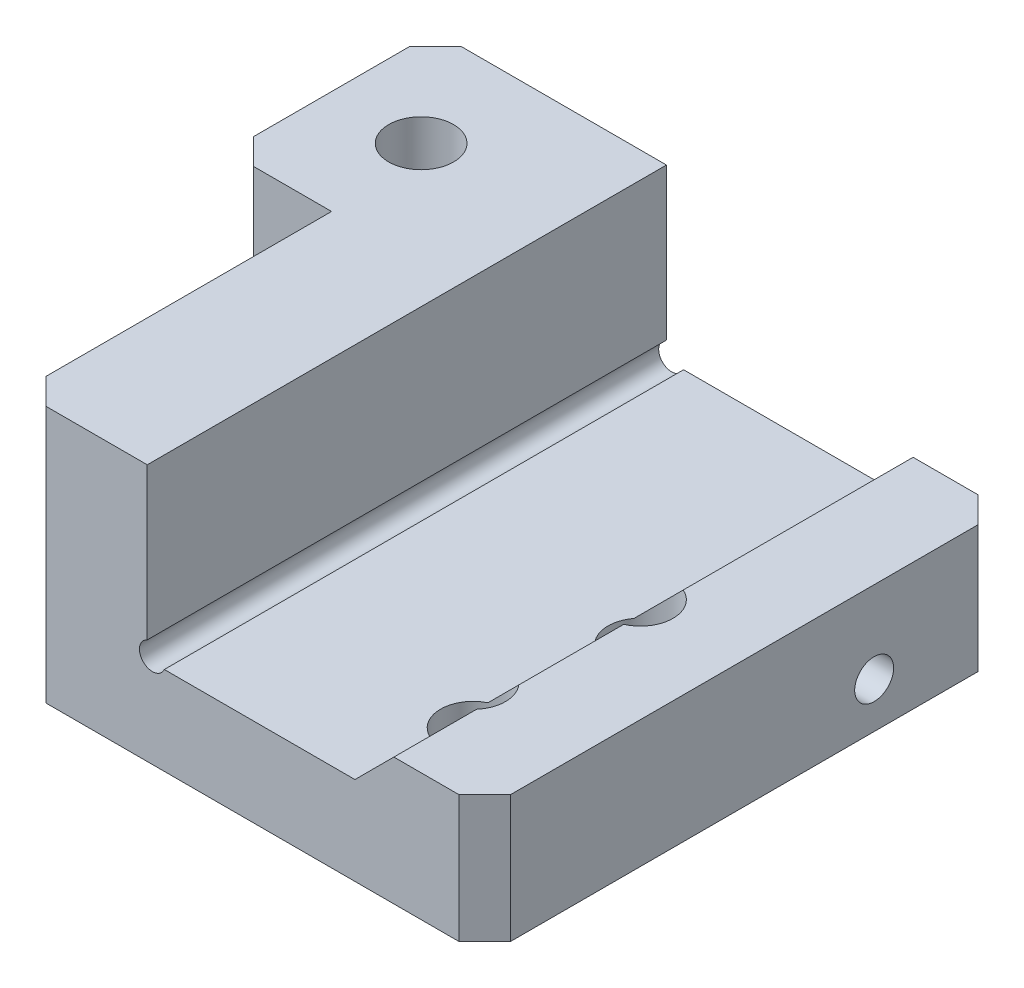
SolidWorks part; units mm, degrees
ref_plane "Front Plane" through (0, 0, 0) normal (0, 0, 1) x (1, 0, 0)
ref_plane "Top Plane" through (0, 0, 0) normal (0, 1, 0) x (1, 0, 0)
ref_plane "Right Plane" through (0, 0, 0) normal (1, 0, 0) x (0, 0, -1)
sketch "Sketch1" plane through (0, 0, 0) normal (0, 0, 1) x (1, 0, 0)
  line L0 (0, 0) -> (0, 6.5)
  line L1 (0, 6.5) -> (4.9, 6.5)
  line L2 (4.9, 6.5) -> (4.9, 4.0583)
  line L3 (5.5583, 3.4) -> (8, 3.4)
  line L4 (8, 3.4) -> (8, 0)
  line L5 (8, 0) -> (0, 0)
  arc A0 (4.9, 4.0583) -> (5.5583, 3.4) centre (5.1, 3.6) ccw
  dimension "D7" = 1
  dimension "D1" = 3.1
  dimension "D2" = 3.1
  dimension "D3" = 6.5
  dimension "D4" = 8
  dimension "D5" = 0.2
  dimension "D6" = 0.2
extrude "Boss-Extrude1" add sketch "Sketch1" along normal blind 20
other "Move Face1" face at (2.45, 6.5, 10) parameters "D1"=3.4
other "Move Face2" face at (8, 1.7, 10) parameters "D1"=9.9
sketch "Sketch10" plane through (0, 0, 0) normal (0, 0, -1) x (-1, 0, 0)
  line L0 (-17.9, 3.4) -> (-17.9, 4.9)
  line L1 (-17.9, 4.9) -> (-14.4, 4.9)
  line L2 (-14.4, 4.9) -> (-12.9, 3.4)
  line L4 (-12.9, 3.4) -> (-17.9, 3.4)
  dimension "D1" = 1.5
  dimension "D2" = 3.5
  dimension "D3" = 45
extrude "Boss-Extrude2" add sketch "Sketch10" against normal up to surface (20 mm away) up to face at (7.2394, 4.3108, 20)
hole_wizard "M3 Tapped Hole1" positions "Sketch11" profile "Sketch12" tap size "M3" standard "GB"
sketch "Sketch11" plane through (0, 0, 0) normal (0, -1, 0) x (-1, 0, 0)
  point P0 (-13.9, -10)
sketch "Sketch12" plane through (13.9, 0, 10) normal (1, 0, 0) x (0, 0, -1)
  line L0 (0, 0) -> (0, 10.7511)
  line L1 (0, 10.7511) -> (1.25, 10)
  line L2 (1.25, 10) -> (1.25, 0)
  line L5 (1.25, 0) -> (0, 0)
  line L10 (0, 10.7511) -> (-1.25, 10) construction
  line L11 (0, -6.35) -> (0, 107.95) construction
  dimension "螺纹孔钻头直径" = 2.5
  dimension "螺纹孔钻头深度" = 10
  dimension "导头角度" = 118
cosmetic thread "Cosmetic thread 2" parameters "D1"=4.9, "D2"=3
sketch "Sketch13" plane through (0, 0, 0) normal (0, -1, 0) x (1, 0, 0)
  line L6 (-4, 8) -> (0, 8)
  line L7 (-4, 8) -> (-4, 0)
  line L8 (-4, 0) -> (0, 0)
  line L9 (0, 8) -> (0, 0)
  line L10 (-4, 8) -> (0, 0) construction
  line L11 (-4, 0) -> (0, 8) construction
  point P0 (-2, 4)
  dimension "D1" = 4
  dimension "D2" = 8
extrude "Boss-Extrude3" add sketch "Sketch13" against normal up to surface (9.9 mm away) up to face at (2.45, 9.9, 10)
hole_wizard "M3 Tapped Hole2" positions "Sketch14" profile "Sketch15" tap size "M3" standard "GB"
sketch "Sketch14" plane through (0, 0, 0) normal (0, -1, 0) x (-1, 0, 0)
  line L2 (-6.45, 0) -> (-6.45, -12.2558) construction
  line L3 (-17.9, -10) -> (-15.3464, -10) construction
  line L4 (-17.9, -20) -> (-17.9, 0) construction
  point P7 (-13.45, -16)
  point P9 (0.55, -4)
  dimension "D1" = 7
  dimension "D2" = 7
  dimension "D3" = 6
  dimension "D4" = 6
sketch "Sketch15" plane through (13.45, 0, 16) normal (1, 0, 0) x (0, 0, -1)
  line L0 (0, 0) -> (0, 10.7511)
  line L1 (0, 10.7511) -> (1.25, 10)
  line L2 (1.25, 10) -> (1.25, 0)
  line L5 (1.25, 0) -> (0, 0)
  line L10 (0, 10.7511) -> (-1.25, 10) construction
  line L11 (0, -6.35) -> (0, 107.95) construction
  dimension "螺纹孔钻头直径" = 2.5
  dimension "螺纹孔钻头深度" = 10
  dimension "导头角度" = 118
cosmetic thread "Cosmetic thread 3" parameters "D1"=6, "D2"=3
cosmetic thread "Cosmetic thread 4" parameters "D1"=4.9, "D2"=3
chamfer "Chamfer1" distance 1 angle 45 5 edges at (17.9, 2.45, 0) (17.9, 2.45, 20) (0, 4.95, 20) (-4, 4.95, 0) (-4, 4.95, 8)
hole_wizard "Size mm dowel hole 0" positions "Sketch17" profile "Sketch18" hole size "Ø1.5" standard "GB"
sketch "Sketch17" plane through (17.9, 0, 0) normal (1, 0, 0) x (0, 0, -1)
  line L2 (-19, 4.9) -> (-1, 4.9) construction
  line L3 (0, 4.9) -> (0, 0) construction
  point P2 (-5, 1.75)
  dimension "D1" = 3.15
  dimension "D2" = 5
sketch "Sketch18" plane through (17.9, 1.75, 5) normal (0, 1, 0) x (0, 0, -1)
  line L0 (0, 0) -> (0, 6.4506)
  line L1 (0, 6.4506) -> (0.75, 6)
  line L2 (0.75, 6) -> (0.75, 0)
  line L5 (0.75, 0) -> (0, 0)
  line L10 (0, 6.4506) -> (-0.75, 6) construction
  line L11 (0, -6.35) -> (0, 107.95) construction
  dimension "孔直径" = 1.5
  dimension "孔深度" = 6
  dimension "导头角度" = 118
